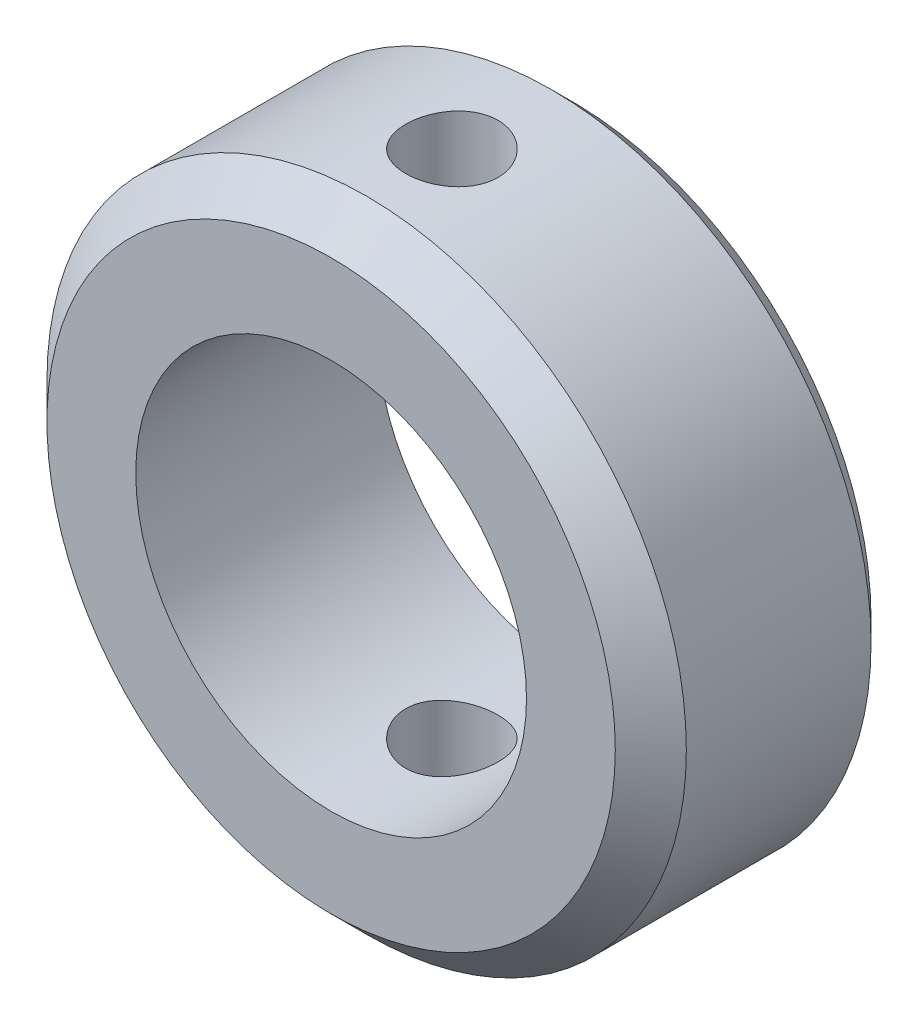
from build123d import *

# Parameters (mm, degrees)
SKETCH1_R               = 45
SKETCH1_R_2             = 27.5
BOSS_EXTRUDE1_DEPTH     = 34
CUT_EXTRUDE1_DEPTH      = 73.15261603
CUT_EXTRUDE1_DEPTH_BACK = 73.15261603
SKETCH3_R               = 6.5
CHAMFER1_SIZE           = 5
CHAMFER2_SIZE           = 3


with BuildPart() as part:
    # Sketch1 → Boss-Extrude1 (new body)
    with BuildSketch(Plane.XY):
        Circle(SKETCH1_R)
        Circle(SKETCH1_R_2, mode=Mode.SUBTRACT)
    extrude(amount=BOSS_EXTRUDE1_DEPTH)

    # Sketch3 → Cut-Extrude1 (cut, two sides: drawn at the far end of the back side and taken through both)
    with BuildSketch(Plane(origin=(0, 0, 0), x_dir=(1, 0, 0), z_dir=(0, 1, 0)).offset(-CUT_EXTRUDE1_DEPTH_BACK)):
        with Locations(Location((0, -17, 0), (0, 0, 270))):
            Circle(SKETCH3_R)
    extrude(amount=CUT_EXTRUDE1_DEPTH + CUT_EXTRUDE1_DEPTH_BACK, mode=Mode.SUBTRACT)

    # Chamfer1
    chamfer1_edges = [part.edges().sort_by_distance(p)[0] for p in [
        (-45, 0, 34),
    ]]
    chamfer(chamfer1_edges, length=CHAMFER1_SIZE)

    # Chamfer2
    chamfer2_edges = [part.edges().sort_by_distance(p)[0] for p in [
        (-45, 0, 0),
    ]]
    chamfer(chamfer2_edges, length=CHAMFER2_SIZE)


solid = part.part
